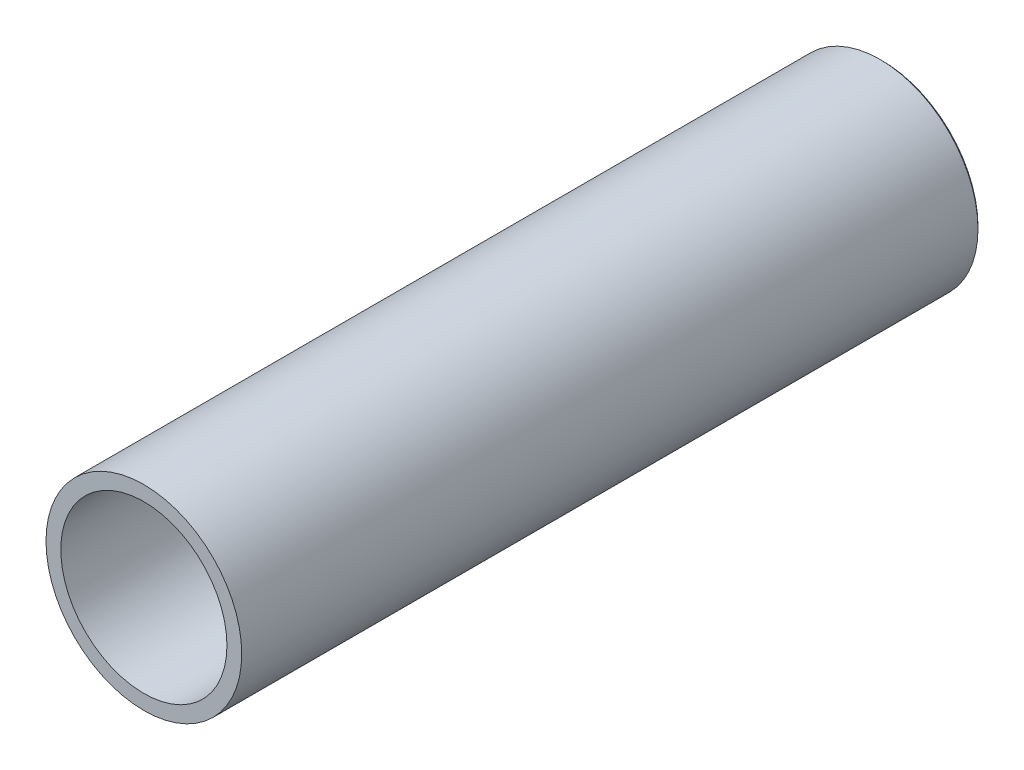
from build123d import *

# Parameters (mm, degrees)
SKETCH_1_R      = 21.2
EXTRUDE_1_DEPTH = 160
SHELL_1_T       = -3.2
CHAMFER_1_SIZE  = 0.5


with BuildPart() as part:
    # 草图1 → 凸台-拉伸1 (new body)
    with BuildSketch(Plane.XY):
        Circle(SKETCH_1_R)
    extrude(amount=EXTRUDE_1_DEPTH)

    # 抽壳1
    shell_1_openings = [part.faces().sort_by_distance(p)[0] for p in [
        (0, 0, 160),
        (0, 0, 0),
    ]]
    offset(amount=SHELL_1_T, openings=shell_1_openings, kind=Kind.INTERSECTION)

    # 倒角1
    chamfer_1_edges = [part.edges().sort_by_distance(p)[0] for p in [
        (-21.2, 0, 0),
    ]]
    chamfer(chamfer_1_edges, length=CHAMFER_1_SIZE)


solid = part.part
